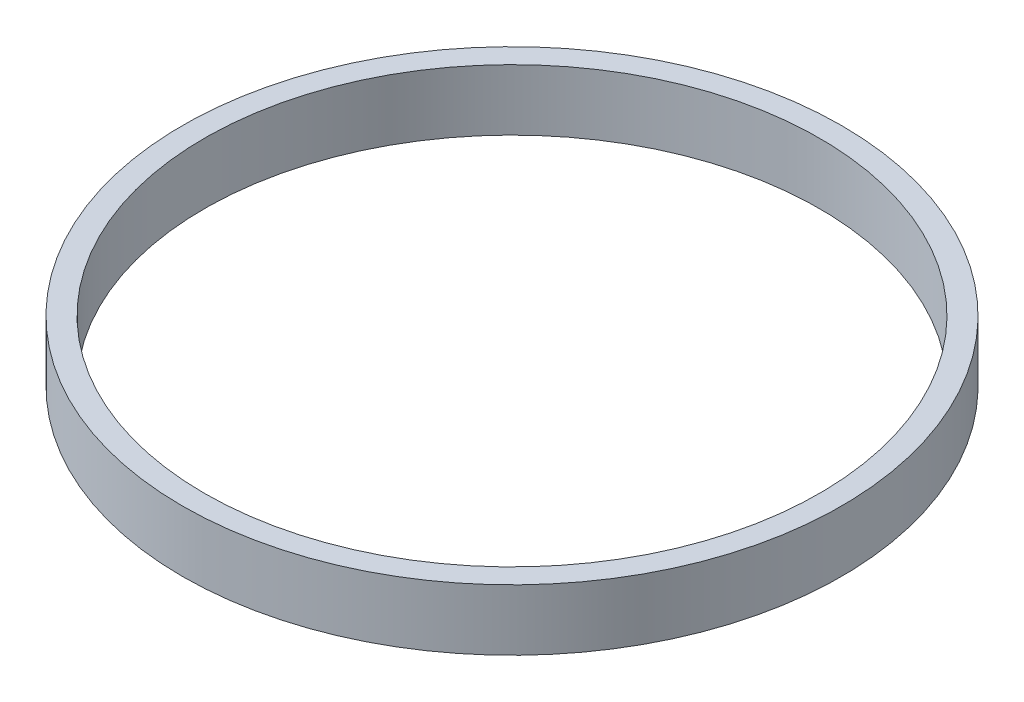
from build123d import *

# Parameters (mm, degrees)
SKETCH1_R           = 13.5
SKETCH1_R_2         = 12.6
BOSS_EXTRUDE1_DEPTH = 2.5


with BuildPart() as part:
    # Sketch1 → Boss-Extrude1 (new body)
    with BuildSketch(Plane(origin=(0, 0, 0), x_dir=(1, 0, 0), z_dir=(0, 1, 0))):
        with Locations(Location((0, 0, 0), (0, 0, 270))):
            Circle(SKETCH1_R)
        with Locations(Location((0, 0, 0), (0, 0, 270))):
            Circle(SKETCH1_R_2, mode=Mode.SUBTRACT)
    extrude(amount=BOSS_EXTRUDE1_DEPTH)


solid = part.part
